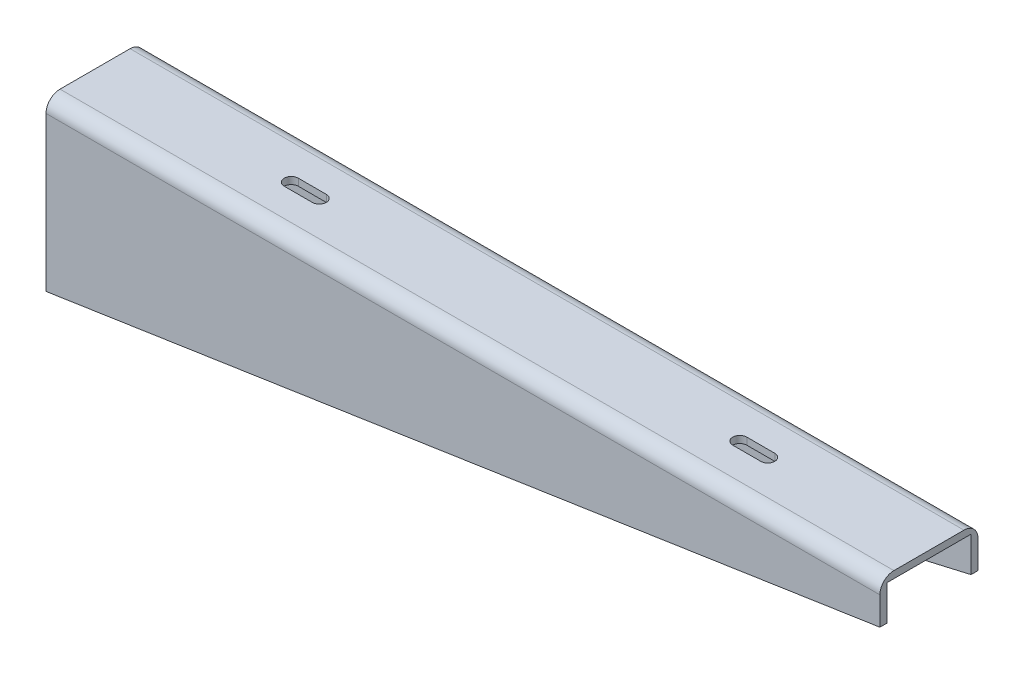
from build123d import *

# Parameters (mm, degrees)
EXTRUDE_1_DEPTH     = 70
SHELL_1_T           = -5
EXTRUDE_2_DEPTH     = 5
CUT_EXTRUDE_1_DEPTH = 5
FILLET_1_R          = 10
FILLET_2_R          = 10
CUT_EXTRUDE_2_DEPTH = 5


with BuildPart() as part:
    # 草图1 → 凸台-拉伸1 (new body)
    with BuildSketch(Plane.XY):
        Polygon((0, 70), (0, -50), (595, 40), (595, 70), (570, 70), align=None)
    extrude(amount=EXTRUDE_1_DEPTH)

    # 抽壳1
    shell_1_openings = [part.faces().sort_by_distance(p)[0] for p in [
        (0, 10, 35),
        (595, 55, 35),
        (297.5, -5, 35),
    ]]
    offset(amount=SHELL_1_T, openings=shell_1_openings, kind=Kind.INTERSECTION)

    # 草图2 → 凸台-拉伸2 (add)
    with BuildSketch(Plane(origin=(0, 0, 0), x_dir=(-1, 0, 0), z_dir=(0, 0, -1))):
        Polygon((-396.666666667, 10), (-595, 40), (-465, 10), align=None)
    extrude(amount=-EXTRUDE_2_DEPTH)

    # 草图3 → 切除-拉伸1 (cut)
    with BuildSketch(Plane(origin=(0, 0, 0), x_dir=(-1, 0, 0), z_dir=(0, 0, -1))):
        Polygon((0, 10), (-396.666666667, 10), (0, -50), align=None)
    extrude(amount=-CUT_EXTRUDE_1_DEPTH, mode=Mode.SUBTRACT)

    # 圆角1
    fillet_1_edges = [part.edges().sort_by_distance(p)[0] for p in [
        (297.5, 70, 0),
    ]]
    fillet(fillet_1_edges, radius=FILLET_1_R)

    # 圆角2
    fillet_2_edges = [part.edges().sort_by_distance(p)[0] for p in [
        (297.5, 70, 70),
    ]]
    fillet(fillet_2_edges, radius=FILLET_2_R)

    # 草图4 → 切除-拉伸2 (cut)
    with BuildSketch(Plane(origin=(0, 70, 0), x_dir=(1, 0, 0), z_dir=(0, 1, 0))):
        with BuildLine():
            Line((460, -30), (480, -30))
            ThreePointArc((480, -30), (485, -35), (480, -40))
            Line((480, -40), (460, -40))
            ThreePointArc((460, -40), (455, -35), (460, -30))
        make_face()
        with BuildLine():
            Line((160, -40), (140, -40))
            ThreePointArc((140, -40), (135, -35), (140, -30))
            Line((140, -30), (160, -30))
            ThreePointArc((160, -30), (165, -35), (160, -40))
        make_face()
    extrude(amount=-CUT_EXTRUDE_2_DEPTH, mode=Mode.SUBTRACT)


solid = part.part
